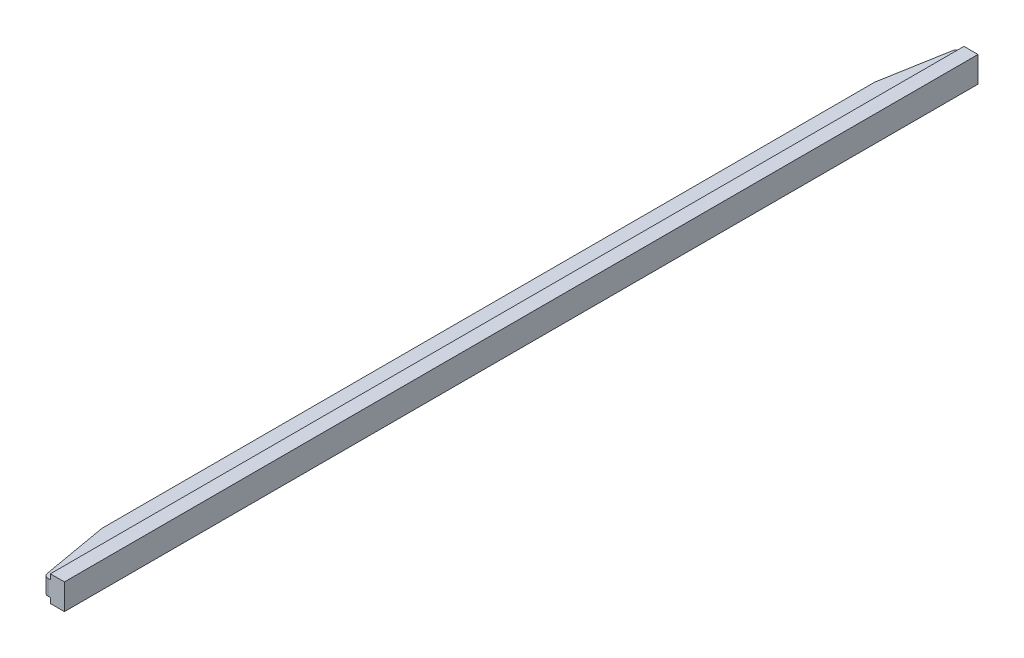
from build123d import *

# Parameters (mm, degrees)
BOSS_EXTRUDE1_DEPTH = 195
CHAMFER1_SIZE       = 30
CHAMFER1_SIZE2      = 5.289809421
FILLET1_R           = 2


with BuildPart() as part:
    # Sketch1 → Boss-Extrude1 (new, symmetric)
    with BuildSketch(Plane.XY):
        Polygon((0, -5.5), (0, 5.5), (-6, 5.5), (-6, 3.3), (-14, 3.3), (-14, -3.3), (-6, -3.3), (-6, -5.5), align=None)
    extrude(amount=BOSS_EXTRUDE1_DEPTH, both=True)

    # Chamfer1
    chamfer1_edges = [part.edges().sort_by_distance(p)[0] for p in [
        (-14, 0, 195),
        (-14, 0, -195),
    ]]
    chamfer1_side = [part.faces().sort_by_distance(p)[0] for p in [
        (-14, 0, 0),
    ]]
    chamfer(chamfer1_edges, length=CHAMFER1_SIZE, length2=CHAMFER1_SIZE2, reference=chamfer1_side[0])

    # Fillet1
    fillet1_edges = [part.edges().sort_by_distance(p)[0] for p in [
        (-14, 0, 165),
        (-14, 0, -165),
        (-8.710190579, 0, -195),
        (-8.710190579, 0, 195),
    ]]
    fillet(fillet1_edges, radius=FILLET1_R)


solid = part.part
